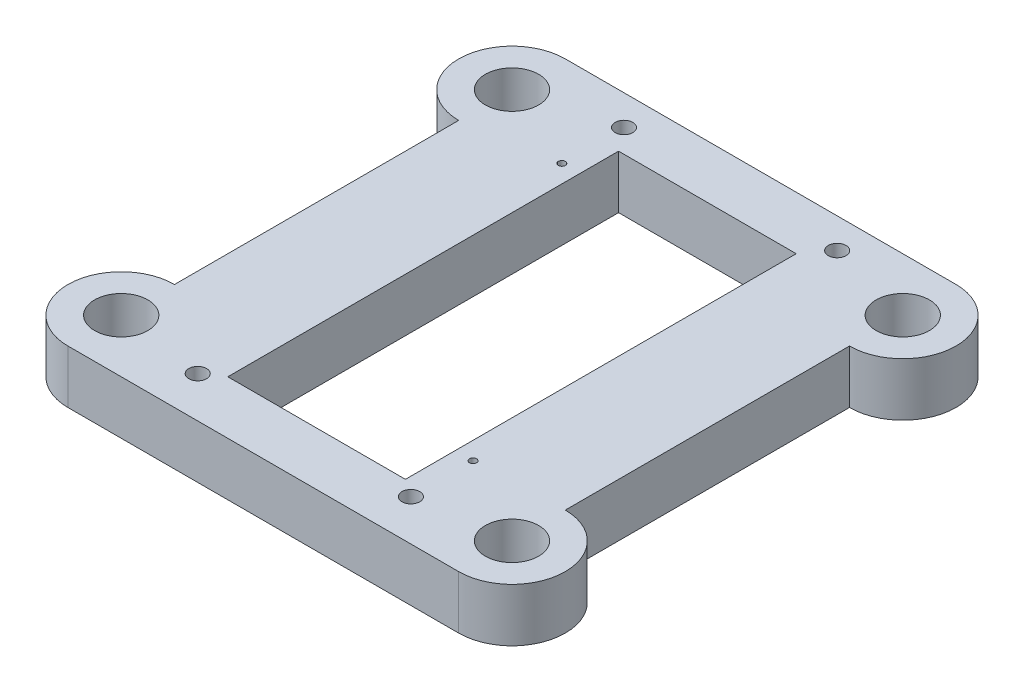
from build123d import *

# Parameters (mm, degrees)
SKETCH1_R                                        = 15
SKETCH1_W                                        = 100
SKETCH1_H                                        = 220
BOSS_EXTRUDE1_DEPTH                              = 30
CBORE_FOR_M8_PAN_HEAD_MACHINE_SCREW3_D           = 9
CBORE_FOR_M8_PAN_HEAD_MACHINE_SCREW3_CBORE_D     = 18
CBORE_FOR_M8_PAN_HEAD_MACHINE_SCREW3_CBORE_DEPTH = 6
SKETCH_1_R                                       = 5
CUT_EXTRUDE1_DEPTH                               = 20
SKETCH2_R                                        = 2
CUT_EXTRUDE2_DEPTH                               = 289.097205818


with BuildPart() as part:
    # Sketch1 → Boss-Extrude1 (new body)
    with BuildSketch(Plane(origin=(0, 0, 0), x_dir=(1, 0, 0), z_dir=(0, 1, 0))):
        with BuildLine():
            Line((-110, -250), (80, -250))
            Line((80, -250), (80, 30))
            Line((80, 30), (-110, 30))
            ThreePointArc((-110, 30), (-140, 0), (-110, -30))
            Line((-110, -30), (-110, -190))
            ThreePointArc((-110, -190), (-140, -220), (-110, -250))
        make_face()
        with Locations(Location((-110, 0, 0), (0, 0, 270))):
            Circle(SKETCH1_R, mode=Mode.SUBTRACT)
        with Locations(Location((-110, -220, 0), (0, 0, 270))):
            Circle(SKETCH1_R, mode=Mode.SUBTRACT)
        with Locations((0, -110)):
            Rectangle(SKETCH1_W, SKETCH1_H, mode=Mode.SUBTRACT)
    boss_extrude1 = extrude(amount=BOSS_EXTRUDE1_DEPTH)

    # CBORE for M8 Pan Head Machine Screw3 (through all)
    with Locations(Plane(origin=(0, 0, 0), x_dir=(-1, 0, 0), z_dir=(0, -1, 0))):
        with Locations((60, -230), (-60, -230), (-60, 10), (60, 10)):
            CounterBoreHole(CBORE_FOR_M8_PAN_HEAD_MACHINE_SCREW3_D / 2, CBORE_FOR_M8_PAN_HEAD_MACHINE_SCREW3_CBORE_D / 2, CBORE_FOR_M8_PAN_HEAD_MACHINE_SCREW3_CBORE_DEPTH)

    # Mirror1: Boss-Extrude1 across plane
    add(boss_extrude1.mirror(Plane(origin=(0, 0, 0), x_dir=(0, 0, 1), z_dir=(1, 0, 0))))

    # 草图1 → Cut-Extrude1 (cut)
    with BuildSketch(Plane(origin=(0, 30, 0), x_dir=(1, 0, 0), z_dir=(0, 1, 0))):
        with Locations(Location((-60, 13.06497659, 0), (0, 0, 270))):
            Circle(SKETCH_1_R)
        with Locations(Location((-60, -226.93502341, 0), (0, 0, 270))):
            Circle(SKETCH_1_R)
        with Locations(Location((60, 13.06497659, 0), (0, 0, 90))):
            Circle(SKETCH_1_R)
        with Locations(Location((60, -226.93502341, 0), (0, 0, 90))):
            Circle(SKETCH_1_R)
    extrude(amount=-CUT_EXTRUDE1_DEPTH, mode=Mode.SUBTRACT)

    # Sketch2 → Cut-Extrude2 (cut, through all)
    with BuildSketch(Plane(origin=(0, 30, 0), x_dir=(1, 0, 0), z_dir=(0, 1, 0))):
        with Locations(Location((-60, -21.93502341, 0), (0, 0, 270))):
            Circle(SKETCH2_R)
        with Locations(Location((60, -191.93502341, 0), (0, 0, 270))):
            Circle(SKETCH2_R)
    extrude(amount=-CUT_EXTRUDE2_DEPTH, mode=Mode.SUBTRACT)


solid = part.part
